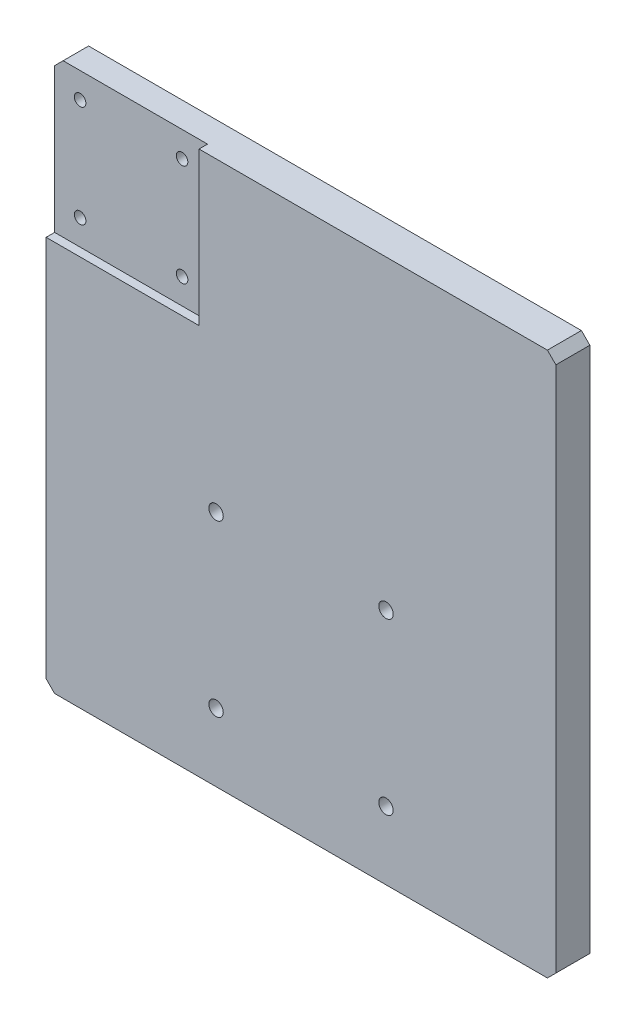
from build123d import *

# Parameters (mm, degrees)
SKETCH_1_W              = 300
SKETCH_1_H              = 320
EXTRUDE_1_DEPTH         = 10
HOLE_WIZARD_M10_1_D     = 8.5
HOLE_WIZARD_M10_1_DEPTH = 15
HOLE_WIZARD_M10_1_TIP   = 2.553657631
SKETCH_7_W              = 90
SKETCH_7_H              = 90
CUT_EXTRUDE_1_DEPTH     = 5
HOLE_WIZARD_M8_1_D      = 6.8
HOLE_WIZARD_M8_1_DEPTH  = 10
HOLE_WIZARD_M8_1_TIP    = 2.042926105
CHAMFER_1_SIZE          = 5


with BuildPart() as part:
    # 草图1 → 凸台-拉伸1 (new, symmetric)
    with BuildSketch(Plane.XY):
        Rectangle(SKETCH_1_W, SKETCH_1_H)
    extrude(amount=EXTRUDE_1_DEPTH, both=True)

    # M10 螺纹孔1
    with Locations(Plane.XY.offset(10)):
        with Locations((50, -20), (-50, -120), (-50, -20), (50, -120)):
            Hole(HOLE_WIZARD_M10_1_D / 2, depth=HOLE_WIZARD_M10_1_DEPTH)
            with Locations((0, 0, -(HOLE_WIZARD_M10_1_DEPTH + HOLE_WIZARD_M10_1_TIP / 2))):  # 118° drill point
                Cone(0, HOLE_WIZARD_M10_1_D / 2, HOLE_WIZARD_M10_1_TIP, mode=Mode.SUBTRACT)

    # 草图7 → 切除-拉伸1 (cut)
    with BuildSketch(Plane.XY.offset(10)):
        with Locations((-105, 115)):
            Rectangle(SKETCH_7_W, SKETCH_7_H)
    extrude(amount=-CUT_EXTRUDE_1_DEPTH, mode=Mode.SUBTRACT)

    # M8 螺纹孔1
    with Locations(Plane.XY.offset(5)):
        with Locations((-75, 85), (-75, 145), (-135, 85), (-135, 145)):
            Hole(HOLE_WIZARD_M8_1_D / 2, depth=HOLE_WIZARD_M8_1_DEPTH)
            with Locations((0, 0, -(HOLE_WIZARD_M8_1_DEPTH + HOLE_WIZARD_M8_1_TIP / 2))):  # 118° drill point
                Cone(0, HOLE_WIZARD_M8_1_D / 2, HOLE_WIZARD_M8_1_TIP, mode=Mode.SUBTRACT)

    # 倒角1
    chamfer_1_edges = [part.edges().sort_by_distance(p)[0] for p in [
        (-150, 160, -2.5),
        (150, -160, 0),
        (-150, -160, 0),
        (150, 160, 0),
    ]]
    chamfer(chamfer_1_edges, length=CHAMFER_1_SIZE)


solid = part.part
